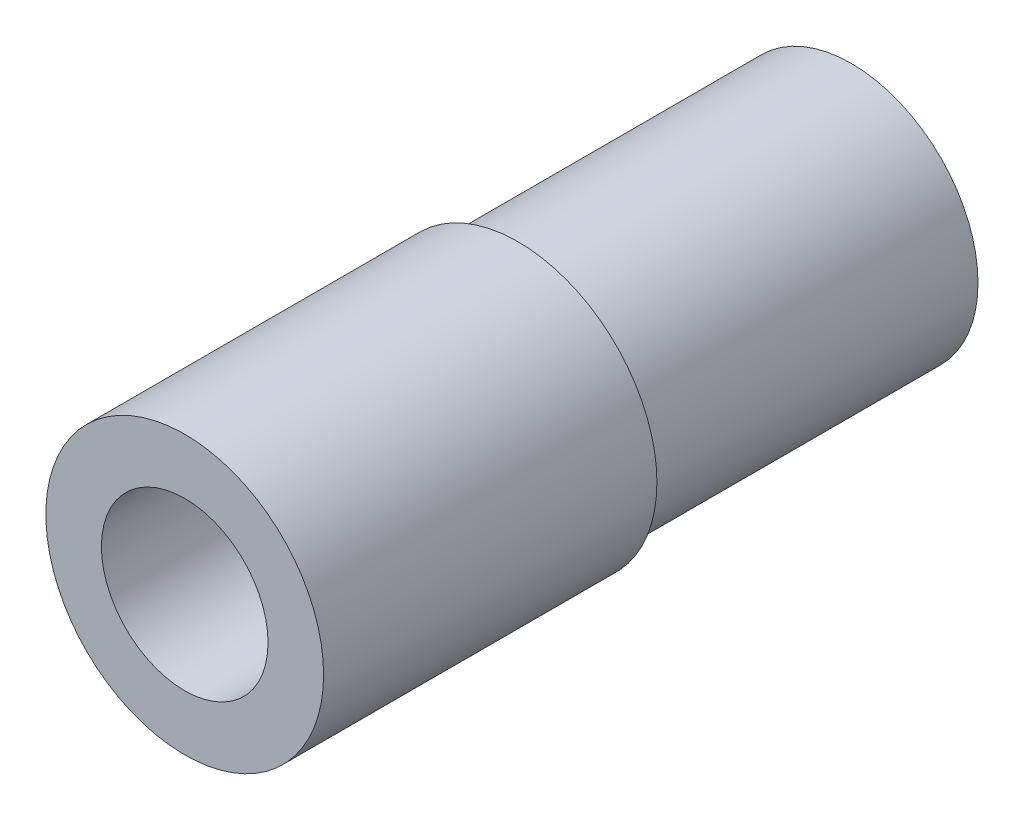
SolidWorks part; units mm, degrees
ref_plane "前视基准面" through (0, 0, 0) normal (0, 0, 1) x (1, 0, 0)
ref_plane "上视基准面" through (0, 0, 0) normal (0, 1, 0) x (1, 0, 0)
ref_plane "右视基准面" through (0, 0, 0) normal (1, 0, 0) x (0, 0, -1)
other "Configuration Table"
sketch "草图1" plane through (0, 0, 0) normal (0, 0, 1) x (1, 0, 0)
  circle A0 centre (0, 0) radius 11.4
  dimension "D1" = 22.8
extrude "凸台-拉伸1" add sketch "草图1" along normal blind 20 and the other way blind 10
cosmetic thread "装饰螺纹线1" parameters "D2"=19.294
sketch "草图2" plane through (0, 0, 20) normal (0, 0, 1) x (1, 0, 0)
  circle A0 centre (0, 0) radius 12.5
  dimension "D1" = 25
extrude "凸台-拉伸2" add sketch "草图2" along normal blind 30
sketch "草图7" plane through (0, 0, 0) normal (1, 0, 0) x (0, 0, -1)
  line L0 (-50, 0) -> (-18, 0)
  line L1 (-50, 12.5) -> (-50, -12.5) construction
  line L2 (-18, 0) -> (-22.5065, 7.5)
  line L3 (-22.5065, 7.5) -> (-50, 7.5)
  line L4 (-50, 7.5) -> (-50, 0)
  dimension "D1" = 7.5
  dimension "D2" = 59
  dimension "D3" = 32
revolve "切除-旋转1" cut sketch "草图7" angle 360 about L0
